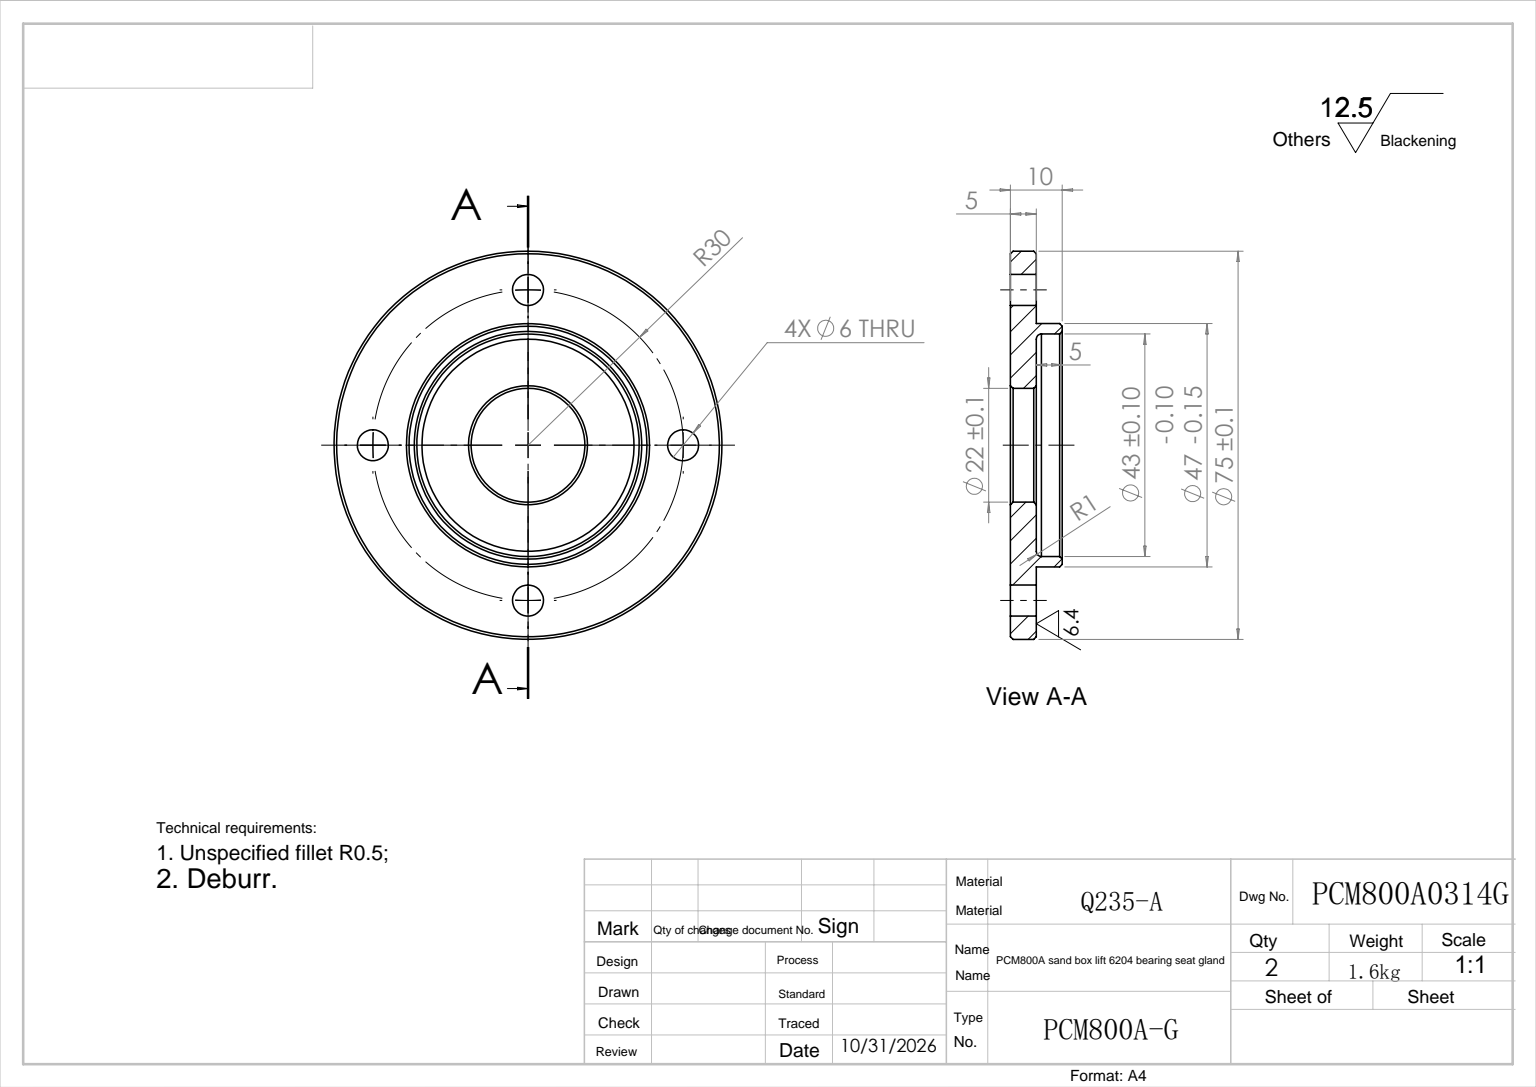
from build123d import *

# Parameters (mm, degrees)
SKETCH_1_R          = 37.5
SKETCH_1_R_2        = 11
EXTRUDE_1_DEPTH     = 5
SKETCH_2_R          = 23.5
SKETCH_2_R_2        = 21.5
EXTRUDE_2_DEPTH     = 5
SKETCH_3_R          = 3
CUT_EXTRUDE_1_DEPTH = 54.967582862
CHAMFER_1_SIZE      = 0.5
FILLET_1_R          = 1
CHAMFER_2_SIZE      = 0.5


with BuildPart() as part:
    # 草图1 → 拉伸1 (new body)
    with BuildSketch(Plane(origin=(0, 0, 0), x_dir=(1, 0, 0), z_dir=(0, 1, 0))):
        with Locations(Location((0, 0, 0), (0, 0, 270))):
            Circle(SKETCH_1_R)
        with Locations(Location((0, 0, 0), (0, 0, 270))):
            Circle(SKETCH_1_R_2, mode=Mode.SUBTRACT)
    extrude(amount=EXTRUDE_1_DEPTH)

    # 草图2 → 拉伸2 (add)
    with BuildSketch(Plane.XZ):
        with Locations(Location((0, 0, 0), (0, 0, 90))):
            Circle(SKETCH_2_R)
        with Locations(Location((0, 0, 0), (0, 0, 270))):
            Circle(SKETCH_2_R_2, mode=Mode.SUBTRACT)
    extrude(amount=EXTRUDE_2_DEPTH)

    # 草图3 → 切除-拉伸1 (cut, through all)
    with BuildSketch(Plane(origin=(0, 5, 0), x_dir=(-1, 0, 0), z_dir=(0, 1, 0))):
        with Locations(Location((-30, 0, 0), (0, 0, 90))):
            Circle(SKETCH_3_R)
        with Locations(Location((0, 30, 0), (0, 0, 90))):
            Circle(SKETCH_3_R)
        with Locations(Location((30, 0, 0), (0, 0, 90))):
            Circle(SKETCH_3_R)
        with Locations(Location((0, -30, 0), (0, 0, 90))):
            Circle(SKETCH_3_R)
    extrude(amount=-CUT_EXTRUDE_1_DEPTH, mode=Mode.SUBTRACT)

    # 倒角1
    chamfer_1_edges = [part.edges().sort_by_distance(p)[0] for p in [
        (0, -5, -23.5),
        (0, -5, 21.5),
        (0, 0, -37.5),
        (0, 5, -37.5),
    ]]
    chamfer(chamfer_1_edges, length=CHAMFER_1_SIZE)

    # 圆角1
    fillet_1_edges = [part.edges().sort_by_distance(p)[0] for p in [
        (0, 0, 21.5),
    ]]
    fillet(fillet_1_edges, radius=FILLET_1_R)

    # 倒角2
    chamfer_2_edges = [part.edges().sort_by_distance(p)[0] for p in [
        (0, 0, -11),
        (0, 5, -11),
    ]]
    chamfer(chamfer_2_edges, length=CHAMFER_2_SIZE)


solid = part.part
